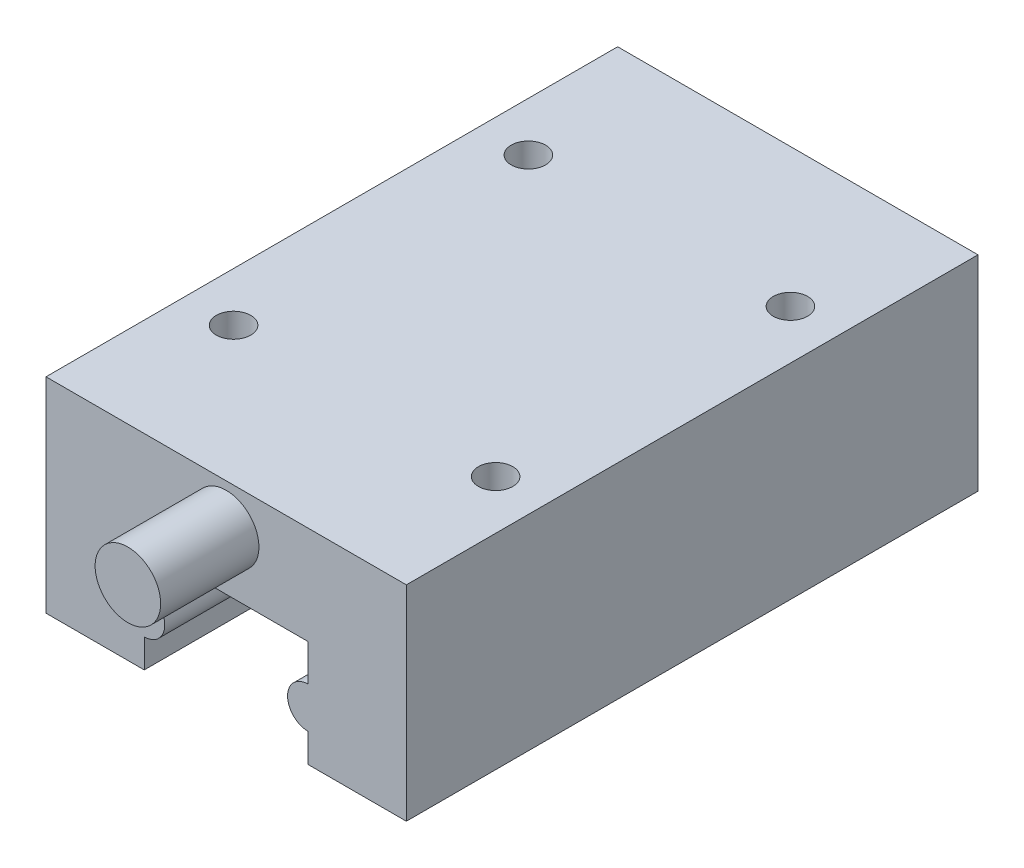
SolidWorks part; units mm, degrees
ref_plane "Front Plane" through (0, 0, 0) normal (0, 0, 1) x (1, 0, 0)
ref_plane "Top Plane" through (0, 0, 0) normal (0, 1, 0) x (1, 0, 0)
ref_plane "Right Plane" through (0, 0, 0) normal (1, 0, 0) x (0, 0, -1)
sketch "Sketch1" plane through (0, 0, 0) normal (0, 0, 1) x (1, 0, 0)
  line L0 (32, -25) -> (44, -25)
  line L1 (0, 0) -> (44, 0)
  line L2 (0, 0) -> (0, -25)
  line L3 (0, -25) -> (12, -25)
  line L4 (44, 0) -> (44, -25)
  line L5 (12, -16.5) -> (12, -12)
  line L6 (12, -25) -> (12, -21.5)
  line L7 (12, -12) -> (32, -12)
  line L8 (32, -25) -> (32, -21.5)
  line L9 (32, -16.5) -> (32, -12)
  arc A0 (12, -21.5) -> (12, -16.5) centre (12, -19) ccw
  arc A1 (32, -16.5) -> (32, -21.5) centre (32, -19) ccw
  dimension "D5" = 5
  dimension "D1" = 44
  dimension "D2" = 25
  dimension "D3" = 20
  dimension "D4" = 13
  dimension "D6" = 6
extrude "Extrude1" add sketch "Sketch1" along normal mid plane 69.8
sketch "Sketch2" plane through (0, 0, 34.9) normal (0, 0, 1) x (1, 0, 0)
  line L0 (44, 0) -> (0, 0) construction
  line L1 (0, 0) -> (0, -25) construction
  circle A0 centre (22, -5) radius 4
  dimension "D1" = 8
  dimension "D2" = 5
  dimension "D3" = 22
extrude "Extrude2" add sketch "Sketch2" along normal blind 12
hole_wizard "M5 Tapped Hole1" positions "3DSketch1" profile "Sketch3" tap size "M5" standard "GB"
sketch3d "3DSketch1"
  line L0 (0, 0, 34.9) -> (0, 0, -34.9) construction
  point P0 (6, 0, 18)
  point P2 (38, 0, 18)
  point P4 (6, 0, -18)
  point P6 (38, 0, -18)
  dimension "D1" = 36
  dimension "D2" = 32
  dimension "D3" = 6
  dimension "D4" = 18
sketch "Sketch3" plane through (6, 0, 18) normal (1, 0, 0) x (0, 0, 1)
  line L0 (0, 0) -> (0, 13.6618)
  line L1 (0, 13.6618) -> (2.1, 12.4)
  line L2 (2.1, 12.4) -> (2.1, 0)
  line L5 (2.1, 0) -> (0, 0)
  line L10 (0, 13.6618) -> (-2.1, 12.4) construction
  line L11 (0, -6.35) -> (0, 107.95) construction
  dimension "螺纹孔钻头直径" = 4.2
  dimension "螺纹孔钻头深度" = 12.4
  dimension "导头角度" = 118
cosmetic thread "Cosmetic Thread5" parameters "D1"=10, "D2"=5
cosmetic thread "Cosmetic Thread6" parameters "D1"=10, "D2"=5
cosmetic thread "Cosmetic Thread7" parameters "D1"=10, "D2"=5
cosmetic thread "Cosmetic Thread8" parameters "D1"=10, "D2"=5
